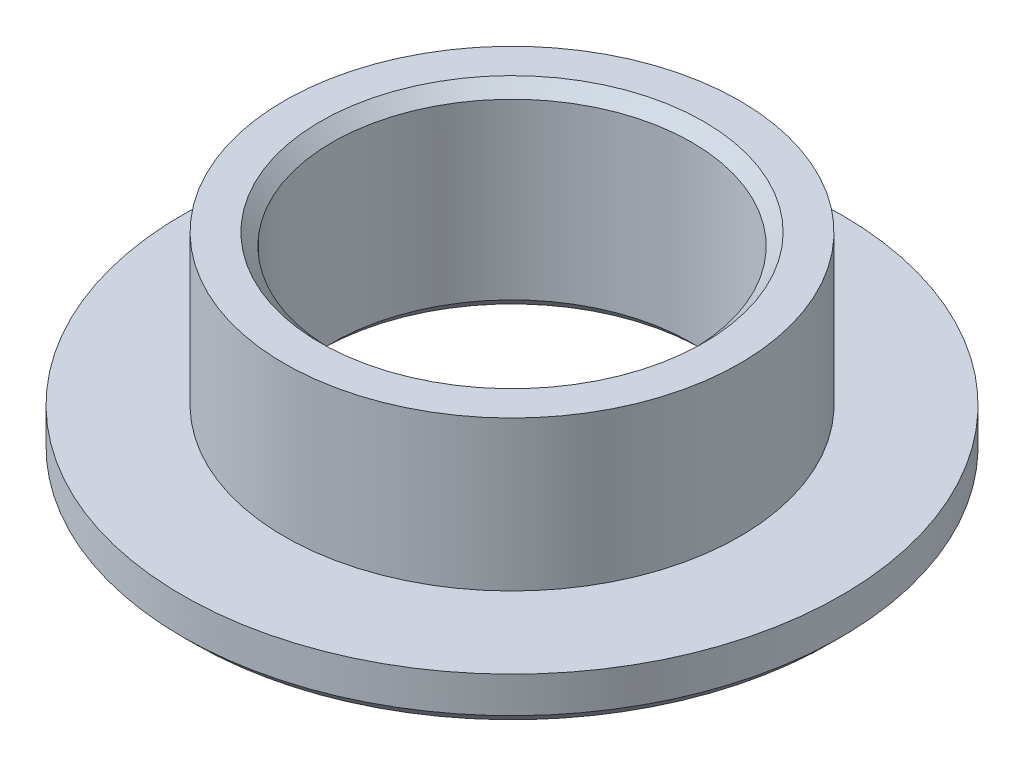
SolidWorks part; units mm, degrees
ref_plane "Front Plane" through (0, 0, 0) normal (0, 0, 1) x (1, 0, 0)
ref_plane "Top Plane" through (0, 0, 0) normal (0, 1, 0) x (1, 0, 0)
ref_plane "Right Plane" through (0, 0, 0) normal (1, 0, 0) x (0, 0, -1)
sketch "Sketch1" plane through (0, 0, 0) normal (0, 0, 1) x (1, 0, 0)
  line L0 (0, 0) -> (0, 76.9475) construction
  line L1 (-30, 0) -> (-30, 33)
  line L2 (-30, 33) -> (-38, 33)
  line L3 (-38, 33) -> (-38, 8)
  line L4 (-38, 8) -> (-55, 8)
  line L5 (-55, 8) -> (-55, 0)
  line L6 (-55, 0) -> (-30, 0)
  dimension "D1" = 30
  dimension "D2" = 38
  dimension "D3" = 55
  dimension "D4" = 33
  dimension "D5" = 25
  dimension "D6" = 8
revolve "Revolve1" add sketch "Sketch1" angle 360 about L0
chamfer "Chamfer1" distance 2 angle 45 3 edges at (0, 0, -55) (0, 33, -30) (0, 0, -30)
